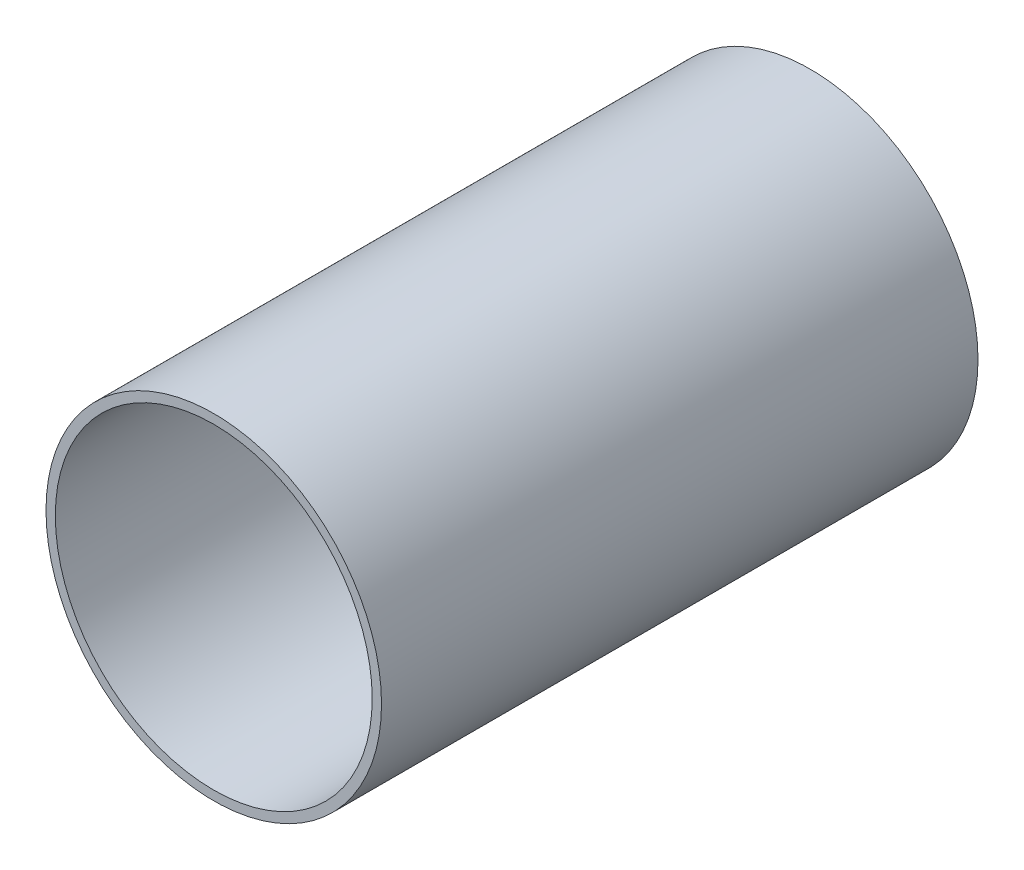
from build123d import *

# Parameters (mm, degrees)
SKETCH_1_R      = 90
SKETCH_1_R_2    = 85
EXTRUDE_2_DEPTH = 320


with BuildPart() as part:
    # 草图1 → 凸台-拉伸2 (new body)
    with BuildSketch(Plane.XY):
        Circle(SKETCH_1_R)
        Circle(SKETCH_1_R_2, mode=Mode.SUBTRACT)
    extrude(amount=EXTRUDE_2_DEPTH)


solid = part.part
